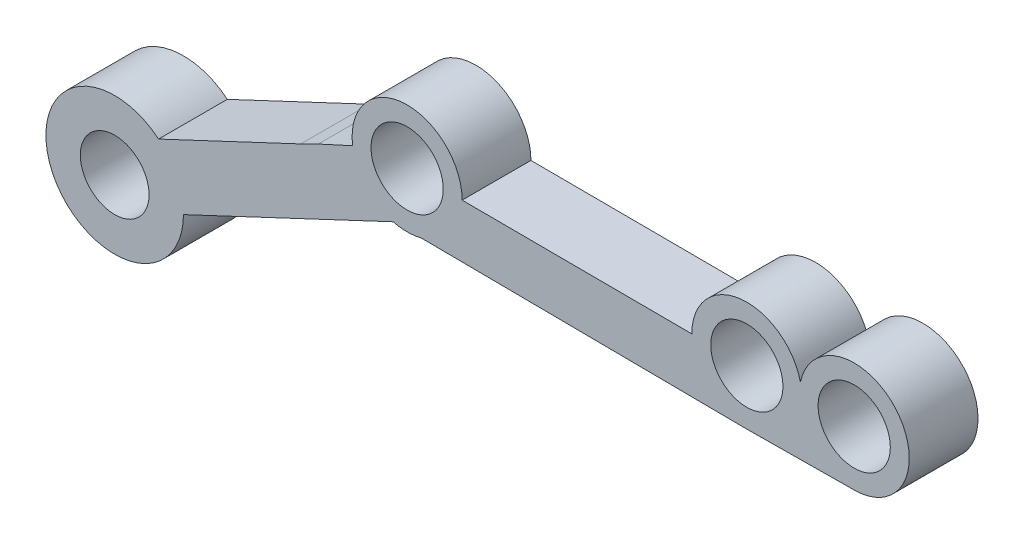
from build123d import *

# Parameters (mm, degrees)
BOSS_EXTRUDE1_DEPTH  = 5
SKETCH3_R            = 2.5
CUT_EXTRUDE3_DEPTH   = 10
SKETCH2_R            = 1.5
CUT_EXTRUDE4_DEPTH   = 7
SKETCH5_R            = 4
BOSS_EXTRUDE2_DEPTH  = 5
SKETCH6_R            = 4
BOSS_EXTRUDE3_DEPTH  = 5
BOSS_EXTRUDE4_DEPTH  = 5
SKETCH9_R            = 4
BOSS_EXTRUDE5_DEPTH  = 5
SKETCH10_R           = 2.625
SKETCH10_R_2         = 2.5
CUT_EXTRUDE5_DEPTH   = 39.359537556
SKETCH11_R           = 4
BOSS_EXTRUDE6_DEPTH  = 5
SKETCH12_R           = 2.625
CUT_EXTRUDE6_DEPTH   = 39.359537556
SKETCH13_R           = 4
BOSS_EXTRUDE7_DEPTH  = 5
CUT_EXTRUDE7_DEPTH   = 39.359537556
CUT_EXTRUDE8_DEPTH   = 39.359537556
BOSS_EXTRUDE8_DEPTH  = 5
BOSS_EXTRUDE9_DEPTH  = 5
CUT_EXTRUDE9_DEPTH   = 10
CUT_EXTRUDE10_DEPTH  = 10
CUT_EXTRUDE11_DEPTH  = 10
CUT_EXTRUDE12_DEPTH  = 10
SKETCH30_R           = 2.5
BOSS_EXTRUDE16_DEPTH = 5


with BuildPart() as part:
    # Sketch1 → Boss-Extrude1 (new body)
    with BuildSketch(Plane.XY):
        with BuildLine():
            Line((0, 0), (34, 0))
            ThreePointArc((34, 0), (34.707106781, -0.292893219), (35, -1))
            Line((35, -1), (35, -4))
            ThreePointArc((35, -4), (34.707106781, -4.707106781), (34, -5))
            Line((34, -5), (0, -5))
            ThreePointArc((0, -5), (-4.600765263, -6.121207346), (-8.169848164, -9.233408201))
            ThreePointArc((-8.169848164, -9.233408201), (-8.772233245, -9.633451101), (-9.486832981, -9.522774425))
            Line((-9.486832981, -9.522774425), (-12.093386622, -8.017879978))
            ThreePointArc((-12.093386622, -8.017879978), (-12.567944885, -7.375988891), (-12.421485667, -6.591272758))
            ThreePointArc((-12.421485667, -6.591272758), (-7.030970465, -1.749888517), (0, 0))
        make_face()
    extrude(amount=BOSS_EXTRUDE1_DEPTH)

    # Sketch3 → Cut-Extrude3 (cut)
    with BuildSketch(Plane(origin=(0, 0, 0), x_dir=(-1, 0, 0), z_dir=(0, 0, -1))):
        with Locations((0, -2.5)):
            Circle(SKETCH3_R)
    extrude(amount=-CUT_EXTRUDE3_DEPTH, mode=Mode.SUBTRACT)


with BuildPart() as cut_extrude3_piece_1:
    # of the separate pieces the step leaves, piece 1, a body of its own (cut_extrude3_pieces)
    add(part.part.solids().sort_by_distance((34, 0, 0))[0])



with BuildPart() as cut_extrude3_piece_2:
    # of the separate pieces the step leaves, piece 2, a body of its own (cut_extrude3_pieces)
    add(part.part.solids().sort_by_distance((-12.421485667, -6.591272758, 0))[0])

    # Sketch2 → Cut-Extrude4 (cut)
    with BuildSketch(Plane.XY.offset(5)):
        with Locations((32.633829537, -2.570962999)):
            Circle(SKETCH2_R)
        with Locations((-9.587088302, -6.686632842)):
            Circle(SKETCH2_R)
        with Locations((24.694851026, -2.570962999)):
            Circle(SKETCH2_R)
    extrude(amount=-CUT_EXTRUDE4_DEPTH, mode=Mode.SUBTRACT)


with BuildPart() as cut_extrude3_piece_1_1:
    add(cut_extrude3_piece_1.part)

    add(cut_extrude3_piece_2.part)  # Boss-Extrude2 merges Cut-Extrude3 piece 2
    # Sketch5 → Boss-Extrude2 (add)
    with BuildSketch(Plane(origin=(0, 0, 0), x_dir=(-1, 0, 0), z_dir=(0, 0, -1))):
        with Locations((0, -2.5)):
            Circle(SKETCH5_R)
    extrude(amount=-BOSS_EXTRUDE2_DEPTH)

    # Sketch6 → Boss-Extrude3 (add, through all)
    with BuildSketch(Plane.XY.offset(5)):
        with Locations((16.69060283, -2.5)):
            Circle(SKETCH6_R)
    extrude(amount=-BOSS_EXTRUDE3_DEPTH)

    # Sketch7 → Boss-Extrude4 (add, through all)
    with BuildSketch(Plane.XY.offset(5)):
        with BuildLine():
            ThreePointArc((29.377501001, -5), (33.824764885, -6.274254628), (36.5, -2.5))
            ThreePointArc((36.5, -2.5), (33.824764885, 1.274254628), (29.377501001, 0))
            Line((29.377501001, 0), (34, 0))
            ThreePointArc((34, 0), (34.707106781, -0.292893219), (35, -1))
            Line((35, -1), (35, -2.5))
            Line((35, -2.5), (35, -4))
            ThreePointArc((35, -4), (34.707106781, -4.707106781), (34, -5))
            Line((34, -5), (29.377501001, -5))
        make_face()
    extrude(amount=-BOSS_EXTRUDE4_DEPTH)

    # Sketch9 → Boss-Extrude5 (add, through all)
    with BuildSketch(Plane.XY.offset(5)):
        with Locations((-9.587088302, -6.686632842)):
            Circle(SKETCH9_R)
    extrude(amount=-BOSS_EXTRUDE5_DEPTH)

    # Sketch10 → Cut-Extrude5 (cut, through all)
    with BuildSketch(Plane.XY.offset(5)):
        with Locations((0, -2.5)):
            Circle(SKETCH10_R)
        with Locations((-9.587088302, -6.686632842)):
            Circle(SKETCH10_R)
        with Locations((16.69060283, -2.5)):
            Circle(SKETCH10_R_2)
        with Locations((32.5, -2.5)):
            Circle(SKETCH10_R)
    extrude(amount=-CUT_EXTRUDE5_DEPTH, mode=Mode.SUBTRACT)

    # Sketch11 → Boss-Extrude6 (add, through all)
    with BuildSketch(Plane.XY.offset(5)):
        with Locations((24.694851026, -2.570962999)):
            Circle(SKETCH11_R)
    extrude(amount=-BOSS_EXTRUDE6_DEPTH)

    # Sketch12 → Cut-Extrude6 (cut, through all)
    with BuildSketch(Plane.XY.offset(5)):
        with Locations((24.694851026, -2.570962999)):
            Circle(SKETCH12_R)
    extrude(amount=-CUT_EXTRUDE6_DEPTH, mode=Mode.SUBTRACT)

    # Sketch13 → Boss-Extrude7 (add, through all)
    with BuildSketch(Plane.XY.offset(5)):
        with Locations((16.69060283, -2.5)):
            Circle(SKETCH13_R)
    extrude(amount=-BOSS_EXTRUDE7_DEPTH)

    # Sketch14 → Cut-Extrude7 (cut, through all)
    with BuildSketch(Plane.XY.offset(5)):
        Polygon((13.568103831, 0), (19.813101829, 0), (19.608152419, 3.101401215), (13.568103831, 2.844182656), (12.582024398, 1.287333479), align=None)
        Polygon((13.568103831, -5), (19.813101829, -5), (20.934648885, -7.644859521), (15.442425287, -9.366014099), (11.632678636, -7.644859521), align=None)
    extrude(amount=-CUT_EXTRUDE7_DEPTH, mode=Mode.SUBTRACT)

    # Sketch15 → Cut-Extrude8 (cut, through all)
    with BuildSketch(Plane.XY.offset(5)):
        Polygon((21.630515983, 0), (5.499420419, 2.191296742), (3.122498999, 0), align=None)
        with BuildLine():
            ThreePointArc((21.630515983, 0), (20.936038702, -1.202997388), (20.694851026, -2.570962999))
            Line((20.694851026, -2.570962999), (4, -2.5))
            ThreePointArc((4, -2.5), (3.774254628, -1.175235115), (3.122498999, 0))
            Line((3.122498999, 0), (21.630515983, 0))
        make_face()
        with BuildLine():
            Line((-7.607535591, 0.794757928), (-3.398220122, -0.39))
            ThreePointArc((-3.398220122, -0.39), (-6.16935857, -1.327435689), (-8.705842203, -2.784914591))
            Line((-8.705842203, -2.784914591), (-7.607535591, 0.794757928))
        make_face()
        with BuildLine():
            ThreePointArc((-3.398220122, -0.39), (-6.16935857, -1.327435689), (-8.705842203, -2.784914591))
            ThreePointArc((-8.705842203, -2.784914591), (-7.460532252, -3.29874864), (-6.456429886, -4.196858178))
            ThreePointArc((-6.456429886, -4.196858178), (-5.240156475, -3.557355191), (-3.961412583, -3.054265596))
            ThreePointArc((-3.961412583, -3.054265596), (-3.913518389, -1.672731107), (-3.398220122, -0.39))
        make_face()
        Polygon((28.45366335, 2.528160998), (29.377501001, 0), (27.75918607, 0), align=None)
        with BuildLine():
            Line((29.377501001, 0), (27.75918607, 0))
            ThreePointArc((27.75918607, 0), (28.271805382, -0.780600595), (28.589454783, -1.658788905))
            ThreePointArc((28.589454783, -1.658788905), (28.886992542, -0.783556844), (29.377501001, 0))
        make_face()
    extrude(amount=-CUT_EXTRUDE8_DEPTH, mode=Mode.SUBTRACT)

    # Sketch16 → Boss-Extrude8 (add, through all)
    with BuildSketch(Plane.XY.offset(5)):
        with BuildLine():
            Line((1.01271432, -6.369678243), (24.694851026, -6.570962999))
            Line((24.694851026, -6.570962999), (32.5, -6.5))
            Line((32.5, -6.5), (28.834380203, -3.557484395))
            Line((28.834380203, -3.557484395), (25.878705121, -5.379005085))
            Line((25.878705121, -5.379005085), (23.335449819, -5.379005085))
            Line((23.335449819, -5.379005085), (21.307719239, -4.244850693))
            Line((21.307719239, -4.244850693), (3.023775712, -3.866799229))
            Line((3.023775712, -3.866799229), (0.570007719, -5.379005085))
            Line((0.570007719, -5.379005085), (-2.853206137, -4.622902157))
            Line((-2.853206137, -4.622902157), (-6.221300997, -5.963266438))
            Line((-6.221300997, -5.963266438), (-6.565043066, -9.307175266))
            ThreePointArc((-6.565043066, -9.307175266), (-3.14075004, -6.897917977), (1.01271432, -6.369678243))
        make_face()
    extrude(amount=-BOSS_EXTRUDE8_DEPTH)

    # Sketch17 → Boss-Extrude9 (add)
    with BuildSketch(Plane(origin=(0, 0, 0), x_dir=(-1, 0, 0), z_dir=(0, 0, -1))):
        Polygon((3.961412583, -3.054265596), (13.495388719, -7.538212462), (11.30366334, -11.209638817), (1.01271432, -6.369678243), align=None)
    extrude(amount=-BOSS_EXTRUDE9_DEPTH)

    # Sketch18 → Cut-Extrude9 (cut)
    with BuildSketch(Plane(origin=(0, 0, 0), x_dir=(-1, 0, 0), z_dir=(0, 0, -1))):
        with BuildLine():
            Line((3.961412583, -3.054265596), (6.456429886, -4.196858178))
            ThreePointArc((6.456429886, -4.196858178), (5.240156475, -3.557355191), (3.961412583, -3.054265596))
        make_face()
    extrude(amount=-CUT_EXTRUDE9_DEPTH, mode=Mode.SUBTRACT)

    # Sketch19 → Cut-Extrude10 (cut)
    with BuildSketch(Plane(origin=(0, 0, 0), x_dir=(-1, 0, 0), z_dir=(0, 0, -1))):
        with BuildLine():
            Line((6.001656968, -8.71603966), (10.116735554, -10.651412003))
            ThreePointArc((10.116735554, -10.651412003), (7.658367525, -10.535986511), (6.001656968, -8.71603966))
        make_face()
    extrude(amount=-CUT_EXTRUDE10_DEPTH, mode=Mode.SUBTRACT)

    # Sketch20 → Cut-Extrude11 (cut)
    with BuildSketch(Plane(origin=(0, 0, 0), x_dir=(-1, 0, 0), z_dir=(0, 0, -1))):
        Polygon((6.456429886, -4.196858178), (7.733220064, -4.828193293), (12.200841034, -6.929370679), (14.105694097, -7.825246628), (14.33213787, -2.397708334), (7.630569976, -1.451472026), align=None)
    extrude(amount=-CUT_EXTRUDE11_DEPTH, mode=Mode.SUBTRACT)

    # Sketch21 → Cut-Extrude12 (cut)
    with BuildSketch(Plane(origin=(0, 0, 0), x_dir=(-1, 0, 0), z_dir=(0, 0, -1))):
        Polygon((11.30366334, -11.209638817), (13.114607064, -7.359126141), (14.222505477, -7.880184465), (12.35401945, -11.85304626), align=None)
    extrude(amount=-CUT_EXTRUDE12_DEPTH, mode=Mode.SUBTRACT)

    # Sketch30 → Boss-Extrude16 (add)
    with BuildSketch(Plane(origin=(0, 0, 0), x_dir=(-1, 0, 0), z_dir=(0, 0, -1))):
        with BuildLine():
            Line((13.114607064, -7.359126141), (11.30366334, -11.209638817))
            Line((11.30366334, -11.209638817), (16.258283795, -13.539858082))
            ThreePointArc((16.258283795, -13.539858082), (25.782858061, -15.668272182), (18.069227519, -9.689345407))
            Line((18.069227519, -9.689345407), (13.114607064, -7.359126141))
        make_face()
        with Locations((21.258283775, -13.540308948)):
            Circle(SKETCH30_R, mode=Mode.SUBTRACT)
    extrude(amount=-BOSS_EXTRUDE16_DEPTH)


solid = cut_extrude3_piece_1_1.part
